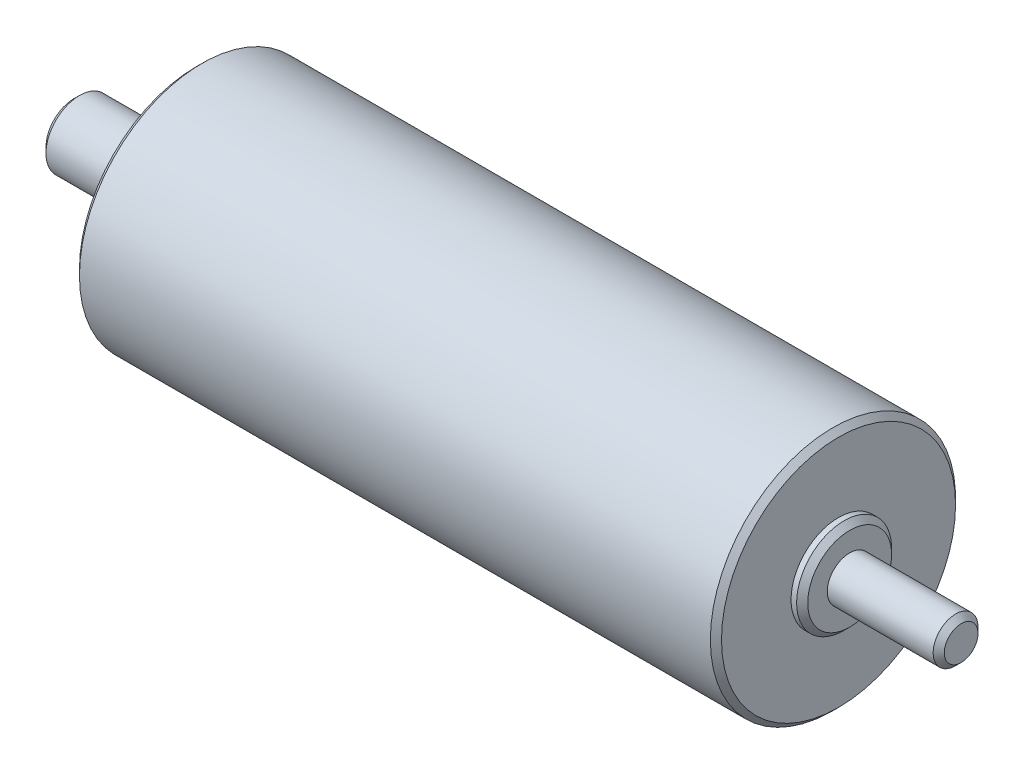
from build123d import *

# Parameters (mm, degrees)
CHAMFER1_SIZE = 0.5


with BuildPart() as part:
    # Sketch1 → Revolve1 (revolve)
    with BuildSketch(Plane.XY, mode=Mode.PRIVATE) as revolve1_sk:
        Polygon((0, 0), (0, 3), (10, 3), (10, 5.25), (11, 5.25), (11, 11), (68.6, 11), (68.6, 4.26180602), (69.6, 4.26180602), (69.6, 2.01180602), (79.6, 2.01180602), (79.6, 0), align=None)
    revolve(revolve1_sk.sketch.rotate(Axis((0, 0, 0), (1, 0, 0)), 90), axis=Axis((0, 0, 0), (1, 0, 0)))

    # Chamfer1
    chamfer1_edges = [part.edges().sort_by_distance(p)[0] for p in [
        (69.6, 0, -4.26180602),
        (68.6, 0, -11),
        (11, 0, -11),
        (10, 0, -5.25),
        (0, 0, -3),
        (79.6, 0, -2.01180602),
    ]]
    chamfer(chamfer1_edges, length=CHAMFER1_SIZE)


solid = part.part
